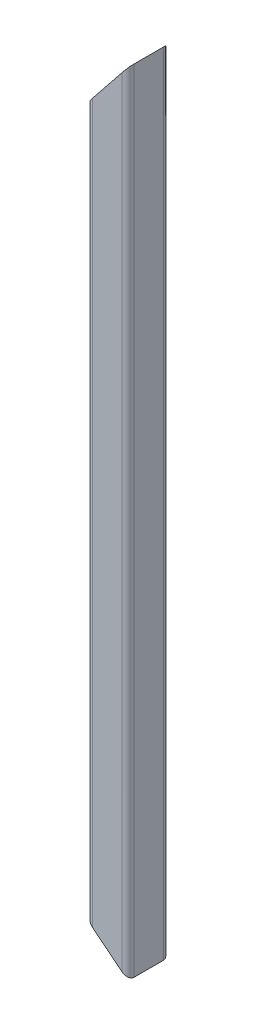
SolidWorks part; units mm, degrees
material "Q235B"
ref_plane "Front Plane" through (0, 0, 0) normal (0, 0, 1) x (1, 0, 0)
ref_plane "Top Plane" through (0, 0, 0) normal (0, 1, 0) x (1, 0, 0)
ref_plane "Right Plane" through (0, 0, 0) normal (1, 0, 0) x (0, 0, -1)
sketch "feature 17 (ProfileFeature) (+16 more in 12 files) Sketch1" plane through (0, 0, 0) normal (0, 0, 1) x (1, 0, 0)
  line L0 (0, 0) -> (0, 1340)
  dimension "D1" = 1340
other "feature 19 (WeldMemberFeat) (+4 more in 5 files) Cold-formed Hollow Structural Square Steel(gb t6728-2002) 70×70×5(1)"
ref_plane "Plane1" through (0, 0, 0) normal (0, 1, 0) x (-1, 0, 0)
sketch "Sketch1" plane through (0, 0, 0) normal (0, 1, 0) x (-1, 0, 0)
  line L0 (-25, -30) -> (25, -30)
  line L1 (-30, -25) -> (-30, 25)
  line L2 (25, 30) -> (-25, 30)
  line L3 (30, 25) -> (30, -25)
  line L4 (-25, -35) -> (25, -35)
  line L5 (-35, -25) -> (-35, 25)
  line L6 (25, 35) -> (-25, 35)
  line L7 (35, 25) -> (35, -25)
  arc A0 (35, 25) -> (25, 35) centre (25, 25) ccw
  arc A1 (25, -35) -> (35, -25) centre (25, -25) ccw
  arc A2 (-35, -25) -> (-25, -35) centre (-25, -25) ccw
  arc A3 (-25, 35) -> (-35, 25) centre (-25, 25) ccw
  arc A4 (-25, 30) -> (-30, 25) centre (-25, 25) ccw
  arc A5 (30, 25) -> (25, 30) centre (25, 25) ccw
  arc A6 (25, -30) -> (30, -25) centre (25, -25) ccw
  arc A7 (-30, -25) -> (-25, -30) centre (-25, -25) ccw
  point P0 (-35, 0)
  point P1 (35, 0)
  point P2 (0, 35)
  point P3 (0, -35)
  point P4 (0, 0)
  point P5 (-35, -35)
  point P6 (35, -35)
  point P7 (35, 35)
  point P8 (-35, 35)
  point P33 (0, 0)
  dimension "D1" = 10
  dimension "D2" = 70
  dimension "D3" = 5
sketch "0:feat:20/0 feature 20/0 (ProfileFeature) (+11 more in 7 files) Sketch2" plane through (0, 0, 35) normal (0, 0, 1) x (1, 0, 0)
  line L0 (35, 1340) -> (-35, 1252.5)
  line L1 (-35, 1340) -> (-35, 0) construction
  line L2 (-35, 1252.5) -> (-35, 1340)
  line L3 (-35, 1340) -> (35, 1340)
  line L4 (-35, 56) -> (35, 0)
  line L5 (35, 0) -> (-35, 0)
  line L6 (-35, 0) -> (-35, 56)
  dimension "D1" = 87.5
  dimension "D2" = 90
extrude "Cut-Extrude1" cut sketch "0:feat:20/0 feature 20/0 (ProfileFeature) (+11 more in 7 files) Sketch2" against normal through all both and the other way through all
